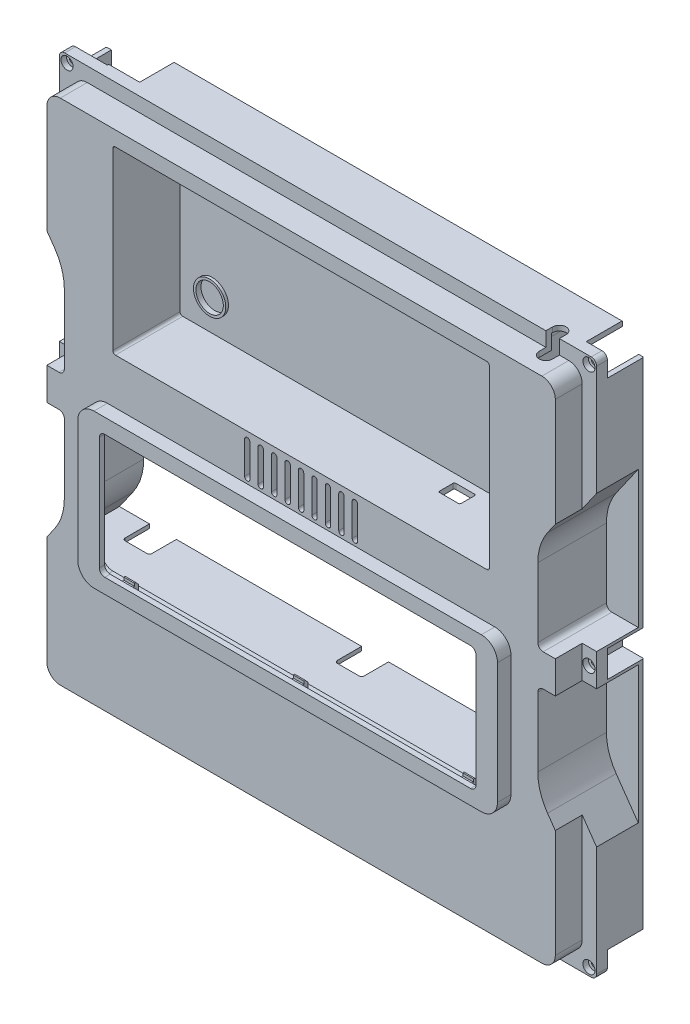
SolidWorks part; units mm, degrees
ref_plane "Front Plane" through (0, 0, 0) normal (0, 0, 1) x (1, 0, 0)
ref_plane "Top Plane" through (0, 0, 0) normal (0, 1, 0) x (1, 0, 0)
ref_plane "Right Plane" through (0, 0, 0) normal (1, 0, 0) x (0, 0, -1)
other "Configuration Table"
sketch "Sketch1" plane through (0, 0, 0) normal (0, 0, 1) x (1, 0, 0)
  line L1 (-100, 100) -> (100, 100)
  line L2 (-100, 100) -> (-100, -100)
  line L3 (-100, -100) -> (100, -100)
  line L4 (100, 100) -> (100, -100)
  line L5 (-100, 100) -> (100, -100) construction
  line L6 (-100, -100) -> (100, 100) construction
  point P0 (0, 0)
  dimension "D1" = 200
  dimension "D2" = 200
extrude "Boss-Extrude1" add sketch "Sketch1" along normal blind 17.5
sketch "Sketch2" plane through (0, 0, 17.5) normal (0, 0, 1) x (1, 0, 0)
  line L1 (-94.5, 94.5) -> (94.5, 94.5)
  line L2 (-94.5, 94.5) -> (-94.5, -94.5)
  line L3 (-94.5, -94.5) -> (94.5, -94.5)
  line L4 (94.5, 94.5) -> (94.5, -94.5)
  line L5 (-94.5, 94.5) -> (94.5, -94.5) construction
  line L6 (-94.5, -94.5) -> (94.5, 94.5) construction
  point P0 (0, 0)
  dimension "D1" = 189
  dimension "D2" = 189
extrude "Boss-Extrude2" add sketch "Sketch2" along normal blind 10
sketch "Sketch3" plane through (0, 0, 27.5) normal (0, 0, 1) x (1, 0, 0)
  line L0 (0, 0) -> (0, 94.5) construction
  line L1 (94.5, 94.5) -> (-94.5, 94.5) construction
  line L2 (-88, 33.694) -> (-88, 6)
  line L3 (-91.617, -45.1656) -> (-112.6112, -75.1484)
  line L4 (-112.6112, -75.1484) -> (-112.6112, 75.1484)
  line L5 (-112.6112, 75.1484) -> (-91.617, 45.1656)
  line L6 (-100, 100) -> (-100, -100) construction
  line L7 (112.6112, 75.1484) -> (91.617, 45.1656)
  line L8 (112.6112, -75.1484) -> (112.6112, 75.1484)
  line L9 (91.617, -45.1656) -> (112.6112, -75.1484)
  line L10 (88, 33.694) -> (88, 6)
  line L11 (-88, 6) -> (-101.9301, 6)
  line L12 (-101.9301, 6) -> (-101.9301, -6)
  line L13 (-101.9301, -6) -> (-88, -6)
  line L14 (-88, -6) -> (-88, -33.694)
  line L15 (101.9301, -6) -> (88, -6)
  line L16 (101.9301, 6) -> (101.9301, -6)
  line L17 (88, 6) -> (101.9301, 6)
  line L18 (88, -6) -> (88, -33.694)
  line L19 (-101.9301, 0) -> (-43.6967, 0) construction
  arc A2 (-88, -33.694) -> (-91.617, -45.1656) centre (-108, -33.694) cw
  arc A3 (-88, 33.694) -> (-91.617, 45.1656) centre (-108, 33.694) ccw
  arc A4 (88, 33.694) -> (91.617, 45.1656) centre (108, 33.694) cw
  arc A5 (88, -33.694) -> (91.617, -45.1656) centre (108, -33.694) ccw
  point P13 (-88, -40)
  point P16 (-88, 40)
  point P25 (88, 40)
  point P26 (88, -40)
  dimension "D5" = 20
  dimension "D1" = 80
  dimension "D2" = 35
  dimension "D3" = 35
  dimension "D4" = 12
  dimension "D6" = 12
  dimension "D7" = 40
extrude "Cut-Extrude2" cut sketch "Sketch3" against normal blind 30
sketch "Sketch4" plane through (0, 0, 27.5) normal (0, 0, 1) x (1, 0, 0)
  line L1 (-69, 89) -> (69, 89)
  line L2 (-70, 88) -> (-70, 23)
  line L3 (-69, 22) -> (69, 22)
  line L4 (70, 88) -> (70, 23)
  line L5 (-70, 89) -> (70, 22) construction
  line L6 (-70, 22) -> (70, 89) construction
  line L7 (-100, -100) -> (100, -100) construction
  arc A0 (69, 22) -> (70, 23) centre (69, 23) ccw
  arc A1 (69, 89) -> (70, 88) centre (69, 88) cw
  arc A2 (-70, 23) -> (-69, 22) centre (-69, 23) ccw
  arc A3 (-69, 89) -> (-70, 88) centre (-69, 88) ccw
  point P0 (0, 55.5)
  dimension "D4" = 1
  dimension "D1" = 67
  dimension "D2" = 140
  dimension "D3" = 122
extrude "Cut-Extrude3" cut sketch "Sketch4" against normal blind 25
sketch "Sketch5" plane through (0, 0, 27.5) normal (0, 0, 1) x (1, 0, 0)
  line L0 (-100, -100) -> (100, -100) construction
  line L1 (-72, 5) -> (72, 5)
  line L2 (-78, -1) -> (-78, -46)
  line L3 (-72, -52) -> (72, -52)
  line L4 (78, -1) -> (78, -46)
  line L5 (-78, 5) -> (78, -52) construction
  line L6 (-78, -52) -> (78, 5) construction
  arc A0 (72, -52) -> (78, -46) centre (72, -46) ccw
  arc A1 (72, 5) -> (78, -1) centre (72, -1) cw
  arc A2 (-78, -46) -> (-72, -52) centre (-72, -46) ccw
  arc A3 (-72, 5) -> (-78, -1) centre (-72, -1) ccw
  point P0 (0, -23.5)
  dimension "D4" = 6
  dimension "D1" = 156
  dimension "D2" = 57
  dimension "D3" = 48
extrude "Boss-Extrude3" add sketch "Sketch5" along normal blind 5
shell "Shell1" thickness 2
sketch "Sketch6" plane through (0, 0, 30.5) normal (0, 0, -1) x (-1, 0, 0)
  line L0 (-72, 3) -> (72, 3) construction
  line L1 (-68, -0.5) -> (68, -0.5)
  line L2 (-70, -2.5) -> (-70, -44.5)
  line L3 (-68, -46.5) -> (68, -46.5)
  line L4 (70, -2.5) -> (70, -44.5)
  line L5 (-70, -0.5) -> (70, -46.5) construction
  line L6 (-70, -46.5) -> (70, -0.5) construction
  arc A0 (-70, -44.5) -> (-68, -46.5) centre (-68, -44.5) ccw
  arc A1 (68, -46.5) -> (70, -44.5) centre (68, -44.5) ccw
  arc A2 (68, -0.5) -> (70, -2.5) centre (68, -2.5) cw
  arc A3 (-68, -0.5) -> (-70, -2.5) centre (-68, -2.5) ccw
  point P0 (0, -23.5)
  dimension "D4" = 2
  dimension "D1" = 140
  dimension "D2" = 46
  dimension "D3" = 3.5
extrude "Cut-Extrude4" cut sketch "Sketch6" against normal through all
sketch "Sketch7" plane through (0, 100, 0) normal (0, 1, 0) x (1, 0, 0)
  line L0 (-88, -10) -> (-79, -10) construction
  line L1 (-88, -8.5) -> (-79, -8.5)
  line L3 (94.5, -17.5) -> (-94.5, -17.5) construction
  line L4 (-100, -17.5) -> (-100, 0) construction
  line L8 (-89.5, -10) -> (-89.5, -13)
  line L9 (100, -17.5) -> (-100, -17.5) construction
  line L10 (-77.5, -10) -> (-77.5, -13)
  line L13 (-89.5, -13) -> (-81, -13)
  line L15 (-77.5, -13) -> (-81, -13)
  arc A0 (-88, -8.5) -> (-89.5, -10) centre (-88, -10) ccw
  arc A1 (-77.5, -10) -> (-79, -8.5) centre (-79, -10) ccw
  point P2 (-85.5, -10.5)
  dimension "D2" = 12
  dimension "D6" = 4.5
  dimension "D1" = 7.5
  dimension "D3" = 9
  dimension "D4" = 4.5
extrude "Cut-Extrude5" cut sketch "Sketch7" against normal blind 5.5
sketch "Sketch9" plane through (0, 0, 27.5) normal (0, 0, 1) x (1, 0, 0)
  line L0 (72, 5) -> (-72, 5) construction
  line L5 (0, 19) -> (0, 7) construction
  line L6 (1, 19) -> (1, 7)
  line L7 (-1, 19) -> (-1, 7)
  arc A0 (1, 19) -> (-1, 19) centre (0, 19) ccw
  arc A1 (-1, 7) -> (1, 7) centre (0, 7) ccw
  point P2 (0, 13)
  dimension "D3" = 2
  dimension "D1" = 2
  dimension "D2" = 12
extrude "Cut-Extrude6" cut sketch "Sketch9" against normal up to next
sketch "Sketch10" plane through (0, 0, 25.5) normal (0, 0, -1) x (-1, 0, 0)
  line L0 (-95.7907, -53.5) -> (-96.5907, -54.3)
  line L1 (95.9105, -53.5) -> (-95.7907, -53.5)
  line L2 (96.7105, -54.3) -> (96.7105, -55)
  line L3 (96.7105, -55) -> (-96.5907, -55)
  line L4 (-96.5907, -54.3) -> (-96.5907, -55)
  line L5 (100, -100) -> (-100, -100) construction
  line L6 (96.7105, -54.3) -> (95.9105, -53.5)
  point P0 (96.7105, -53.5)
  point P3 (-96.5907, -53.5)
  dimension "D1" = 1.5
  dimension "D2" = 45
extrude "Boss-Extrude4" add sketch "Sketch10" along normal blind 25.5
pattern_linear "LPattern1" count 5 spacing 5 along (1, 0, 0) count 5 spacing 5 along (-1, 0, 0) seed only of "Cut-Extrude6"
sketch "Sketch12" plane through (0, 100, 0) normal (0, 1, 0) x (1, 0, 0)
  line L0 (-77.5, -13) -> (-77.5, -10) construction
  line L1 (-77.5, -11.5) -> (-89.5, -11.5)
  line L2 (-77.5, -11.5) -> (-77.5, 7.4305)
  line L3 (-77.5, 7.4305) -> (-89.5, 7.4305)
  line L4 (-89.5, -11.5) -> (-89.5, 7.4305)
extrude "Cut-Extrude8" cut sketch "Sketch12" against normal blind 2
sketch "Sketch13" plane through (0, 0, 2.5) normal (0, 0, 1) x (1, 0, 0)
  line L0 (-70, 55.5) -> (70, 55.5) construction
  line L1 (-70, 88) -> (-70, 23) construction
  line L2 (70, 23) -> (70, 88) construction
  line L3 (0, 89) -> (0, 22) construction
  line L4 (69, 89) -> (-69, 89) construction
  line L5 (-69, 22) -> (69, 22) construction
  line L6 (69, 89) -> (-69, 89) construction
  line L7 (-58, 77) -> (58, 77) construction
  line L8 (-58, 77) -> (-58, 34) construction
  line L9 (-58, 34) -> (58, 34) construction
  line L10 (58, 77) -> (58, 34) construction
  line L11 (-58, 77) -> (58, 34) construction
  line L12 (-58, 34) -> (58, 77) construction
  circle A0 centre (-58, 77) radius 5.1
  circle A1 centre (58, 77) radius 5.1
  circle A2 centre (58, 34) radius 5.1
  circle A3 centre (-58, 34) radius 5.1
  circle A4 centre (-58, 77) radius 6
  circle A5 centre (-58, 34) radius 6
  circle A6 centre (58, 34) radius 6
  circle A7 centre (58, 77) radius 6
  point P12 (0, 55.5)
  dimension "D1" = 12
  dimension "D2" = 10.2
  dimension "D3" = 12
  dimension "D4" = 12
extrude "Boss-Extrude5" add sketch "Sketch13" along normal blind 1
sketch "Sketch14" plane through (0, 0, 0) normal (0, 0, -1) x (-1, 0, 0)
  line L1 (92, 108) -> (108, 108)
  line L2 (92, 108) -> (92, 92)
  line L3 (92, 92) -> (108, 92)
  line L4 (108, 108) -> (108, 92)
  line L5 (92, 108) -> (108, 92) construction
  line L6 (92, 92) -> (108, 108) construction
  line L7 (-108, 108) -> (-92, 108)
  line L8 (-108, 108) -> (-108, 92)
  line L9 (-108, 92) -> (-92, 92)
  line L10 (-92, 108) -> (-92, 92)
  line L11 (-108, 108) -> (-92, 92) construction
  line L12 (-108, 92) -> (-92, 108) construction
  line L13 (92, -92) -> (108, -92)
  line L14 (92, -92) -> (92, -108)
  line L15 (92, -108) -> (108, -108)
  line L16 (108, -92) -> (108, -108)
  line L17 (92, -92) -> (108, -108) construction
  line L18 (92, -108) -> (108, -92) construction
  line L19 (-108, -92) -> (-92, -92)
  line L20 (-108, -92) -> (-108, -108)
  line L21 (-108, -108) -> (-92, -108)
  line L22 (-92, -92) -> (-92, -108)
  line L23 (-108, -92) -> (-92, -108) construction
  line L24 (-108, -108) -> (-92, -92) construction
  line L25 (100, 100) -> (100, 57.1378) construction
  line L26 (89.5, 100) -> (100, 100) construction
  line L27 (-100, -100) -> (-100, -57.1378) construction
  line L28 (100, -100) -> (-100, -100) construction
  line L30 (-110.1437, 10.9337) -> (-92, 10.9337)
  line L31 (-110.1437, 10.9337) -> (-110.1437, -10.1129)
  line L32 (-110.1437, -10.1129) -> (-92, -10.1129)
  line L33 (-92, 10.9337) -> (-92, -10.1129)
  line L34 (92, 13.3418) -> (106.1151, 13.3418)
  line L35 (92, 13.3418) -> (92, -10.1129)
  line L36 (92, -10.1129) -> (106.1151, -10.1129)
  line L37 (106.1151, 13.3418) -> (106.1151, -10.1129)
  point P0 (100, 100)
  point P6 (-100, 100)
  point P12 (100, -100)
  point P18 (-100, -100)
  dimension "D1" = 8
  dimension "D2" = 8
  dimension "D3" = 8
  dimension "D4" = 8
extrude "Cut-Extrude9" cut sketch "Sketch14" against normal blind 13.5
sketch "Sketch15" plane through (0, 0, 15.5) normal (0, 0, -1) x (-1, 0, 0)
  line L0 (92.5, -92.5) -> (-92.5, -92.5) construction
  line L1 (-98, 98) -> (-92.5, 98)
  line L2 (-98, 98) -> (-98, 92.5)
  line L3 (-98, 92.5) -> (-92.5, 92.5)
  line L4 (-92.5, 98) -> (-92.5, 92.5)
  line L5 (98, 98) -> (92.5, 98)
  line L6 (98, 98) -> (98, 92.5)
  line L7 (98, 92.5) -> (92.5, 92.5)
  line L8 (92.5, 98) -> (92.5, 92.5)
  line L9 (98, -98) -> (92.5, -98)
  line L10 (98, -98) -> (98, -92.5)
  line L11 (98, -92.5) -> (92.5, -92.5)
  line L12 (92.5, -98) -> (92.5, -92.5)
  line L13 (-98, -98) -> (-92.5, -98)
  line L14 (-98, -98) -> (-98, -92.5)
  line L15 (-98, -92.5) -> (-92.5, -92.5)
  line L16 (-92.5, -98) -> (-92.5, -92.5)
  line L17 (92.5, -92.5) -> (-92.5, -92.5) construction
  line L19 (-100, 6) -> (-92, 6)
  line L20 (-100, 6) -> (-100, -6)
  line L21 (-100, -6) -> (-92, -6)
  line L22 (-92, 6) -> (-92, -6)
  line L23 (100, 6) -> (92, 6)
  line L24 (100, 6) -> (100, -6)
  line L25 (100, -6) -> (92, -6)
  line L26 (92, 6) -> (92, -6)
extrude "Boss-Extrude6" add sketch "Sketch15" along normal blind 2
sketch "Sketch16" plane through (0, 0, 17.5) normal (0, 0, 1) x (1, 0, 0)
  line L0 (94.5, -94.5) -> (94.5, -55) construction
  line L1 (-97, 97) -> (97, 97) construction
  line L2 (-97, 97) -> (-97, -97) construction
  line L3 (-97, -97) -> (97, -97) construction
  line L4 (97, 97) -> (97, -97) construction
  line L5 (-94.5, -94.5) -> (94.5, -94.5) construction
  line L6 (94.5, 94.5) -> (-94.5, 94.5) construction
  line L7 (-94.5, 94.5) -> (-94.5, 49.283) construction
  circle A0 centre (-97, 97) radius 1.1
  circle A1 centre (97, 97) radius 1.1
  circle A2 centre (97, -97) radius 1.1
  circle A3 centre (-97, -97) radius 1.1
  circle A4 centre (-97, 0) radius 1.1
  circle A5 centre (97, 0) radius 1.1
  dimension "D5" = 2.2
  dimension "D1" = 2.5
  dimension "D2" = 2.5
  dimension "D3" = 2.5
  dimension "D4" = 2.5
extrude "Cut-Extrude10" cut sketch "Sketch16" against normal through all
sketch "Sketch17" plane through (0, 0, 0) normal (0, 0, -1) x (-1, 0, 0)
  line L1 (86, 4) -> (92, 4)
  line L2 (86, 4) -> (86, -4)
  line L3 (86, -4) -> (92, -4)
  line L4 (92, 4) -> (92, -4)
  line L5 (-92, 4) -> (-86, 4)
  line L6 (-92, 4) -> (-92, -4)
  line L7 (-92, -4) -> (-86, -4)
  line L8 (-86, 4) -> (-86, -4)
extrude "Boss-Extrude7" add sketch "Sketch17" against normal blind 16
sketch "Sketch18" plane through (0, 0, 27.5) normal (0, 0, 1) x (1, 0, 0)
  line L0 (100, -100) -> (100, -57.1378) construction
  line L1 (-99.85, 99.85) -> (99.85, 99.85)
  line L2 (-99.85, 99.85) -> (-99.85, -99.85)
  line L3 (-99.85, -99.85) -> (99.85, -99.85)
  line L4 (99.85, 99.85) -> (99.85, -99.85)
  line L5 (-100, -100) -> (100, -100) construction
  line L6 (100, 100) -> (-100, 100) construction
  line L7 (-100, 100) -> (-100, 57.1378) construction
  line L9 (-153.5512, 137.0974) -> (153.5512, 137.0974)
  line L10 (-153.5512, 137.0974) -> (-153.5512, -137.0974)
  line L11 (-153.5512, -137.0974) -> (153.5512, -137.0974)
  line L12 (153.5512, 137.0974) -> (153.5512, -137.0974)
  line L13 (-153.5512, 137.0974) -> (153.5512, -137.0974) construction
  line L14 (-153.5512, -137.0974) -> (153.5512, 137.0974) construction
  point P12 (0, 0)
  dimension "D1" = 0.15
  dimension "D2" = 0.15
  dimension "D3" = 0.15
  dimension "D4" = 0.15
extrude "Cut-Extrude11" cut sketch "Sketch18" against normal through all both and the other way through all
sketch "Sketch20" plane through (0, 99.85, 0) normal (0, 1, 0) x (1, 0, 0)
  line L1 (-86, -13.5) -> (-98, -13.5)
  line L2 (-86, -13.5) -> (-86, 0)
  line L3 (-86, 0) -> (-98, 0)
  line L4 (-98, -13.5) -> (-98, 0)
extrude "Cut-Extrude12" cut sketch "Sketch20" against normal up to next and the other way through all
sketch "Sketch22" plane through (0, 0, 25.5) normal (0, 0, -1) x (-1, 0, 0)
  line L0 (-26, 20) -> (-26, 8)
  line L1 (69, 20) -> (-69, 20) construction
  line L2 (-24, 6) -> (24, 6)
  line L3 (26, 8) -> (26, 20)
  line L4 (69, 20) -> (20, 20) construction
  line L6 (-27, 20) -> (-27, 8)
  line L7 (-24, 5) -> (24, 5)
  line L8 (27, 8) -> (27, 20)
  line L9 (-27, 20) -> (-26, 20)
  line L10 (26, 20) -> (27, 20)
  line L11 (68, -0.5) -> (-68, -0.5) construction
  arc A0 (24, 6) -> (26, 8) centre (24, 8) ccw
  arc A1 (-26, 8) -> (-24, 6) centre (-24, 8) ccw
  arc A2 (-27, 8) -> (-24, 5) centre (-24, 8) ccw
  arc A3 (24, 5) -> (27, 8) centre (24, 8) ccw
  point P13 (26, 4)
  point P16 (-26, 4)
  dimension "D4" = 2
  dimension "D7" = 26
  dimension "D8" = 3
  dimension "D9" = 3
  dimension "D1" = 1
  dimension "D2" = 26
  dimension "D3" = 5.5
  dimension "D5" = 1
  dimension "D6" = 1
extrude "Boss-Extrude8" add sketch "Sketch22" along normal blind 12
sketch "Sketch23" plane through (0, 20, 0) normal (0, -1, 0) x (-1, 0, 0)
  line L0 (69, -25.5) -> (27, -25.5) construction
  line L1 (-42.5, -5.5) -> (-35.5, -5.5)
  line L2 (-43, -6) -> (-43, -11)
  line L3 (-42.5, -11.5) -> (-35.5, -11.5)
  line L4 (-35, -6) -> (-35, -11)
  line L5 (-43, -5.5) -> (-35, -11.5) construction
  line L6 (-43, -11.5) -> (-35, -5.5) construction
  line L7 (-26, -13.5) -> (-26, -25.5) construction
  arc A0 (-35.5, -5.5) -> (-35, -6) centre (-35.5, -6) cw
  arc A1 (-35.5, -11.5) -> (-35, -11) centre (-35.5, -11) ccw
  arc A2 (-43, -11) -> (-42.5, -11.5) centre (-42.5, -11) ccw
  arc A3 (-42.5, -5.5) -> (-43, -6) centre (-42.5, -6) ccw
  point P0 (-39, -8.5)
  dimension "D5" = 0.5
  dimension "D1" = 8
  dimension "D2" = 6
  dimension "D3" = 14
  dimension "D4" = 9
extrude "Cut-Extrude14" cut sketch "Sketch23" against normal up to next
sketch "Sketch24" plane through (0, -55, 0) normal (0, -1, 0) x (-1, 0, 0)
  line L0 (-96.0616, 0) -> (96.0616, 0) construction
  line L1 (5, 10) -> (-5, 10)
  line L2 (5, 10) -> (5, -9)
  line L3 (4, -10) -> (-4, -10)
  line L4 (-5, 10) -> (-5, -9)
  line L5 (5, 10) -> (-5, -10) construction
  line L6 (5, -10) -> (-5, 10) construction
  line L7 (0, 0) -> (0, 21.535) construction
  line L8 (-83.8576, 9.6048) -> (-73.8576, 9.6048)
  line L9 (-83.8576, 9.6048) -> (-83.8576, -9)
  line L10 (-82.8576, -10) -> (-74.8576, -10)
  line L11 (-73.8576, 9.6048) -> (-73.8576, -9)
  line L12 (73.8576, 9.6048) -> (73.8576, -9)
  line L13 (82.8576, -10) -> (74.8576, -10)
  line L14 (83.8576, 9.6048) -> (83.8576, -9)
  line L15 (83.8576, 9.6048) -> (73.8576, 9.6048)
  arc A0 (-4, -10) -> (-5, -9) centre (-4, -9) cw
  arc A1 (5, -9) -> (4, -10) centre (4, -9) cw
  arc A2 (-74.8576, -10) -> (-73.8576, -9) centre (-74.8576, -9) ccw
  arc A3 (-83.8576, -9) -> (-82.8576, -10) centre (-82.8576, -9) ccw
  arc A4 (83.8576, -9) -> (82.8576, -10) centre (82.8576, -9) cw
  arc A5 (74.8576, -10) -> (73.8576, -9) centre (74.8576, -9) cw
  point P0 (0, 0)
  point P20 (-73.8576, -10)
  point P23 (-83.8576, -10)
  point P34 (83.8576, -10)
  point P35 (73.8576, -10)
  dimension "D3" = 1
  dimension "D5" = 1
  dimension "D1" = 10
  dimension "D2" = 10
  dimension "D4" = 10
extrude "Cut-Extrude15" cut sketch "Sketch24" against normal up to next
sketch "Sketch25" plane through (0, 0, 30.5) normal (0, 0, -1) x (-1, 0, 0)
  line L0 (0, 0) -> (0, -21.9735) construction
  line L5 (-65, 2.5) -> (65, 2.5)
  line L6 (-65, 2.5) -> (-65, 1)
  line L7 (-65, 1) -> (65, 1)
  line L8 (65, 2.5) -> (65, 1)
  line L9 (-65, 2.5) -> (65, 1) construction
  line L10 (-65, 1) -> (65, 2.5) construction
  line L15 (-68, -46.5) -> (68, -46.5) construction
  line L16 (65, -49.5) -> (-65, -49.5)
  line L17 (-70, -23.5) -> (27.1802, -23.5) construction
  line L18 (-70, -2.5) -> (-70, -44.5) construction
  line L19 (68, -0.5) -> (-68, -0.5) construction
  line L20 (65, -49.5) -> (65, -48)
  line L21 (65, -48) -> (-65, -48)
  line L26 (-65, -49.5) -> (-65, -48)
  line L27 (65, -49.5) -> (-65, -48) construction
  line L28 (65, -48) -> (-65, -49.5) construction
  point P4 (0, 1.75)
  point P9 (0, -48.75)
  dimension "D1" = 1.5
  dimension "D2" = 1.5
  dimension "D3" = 130
  dimension "D4" = 1.5
  dimension "D5" = 1.5
extrude "Boss-Extrude9" add sketch "Sketch25" along normal blind 2.1
sketch "Sketch26" plane through (-65, 0, 0) normal (-1, 0, 0) x (0, 0, 1)
  line L0 (28.4, 1) -> (28.4, 0)
  line L1 (28.4, 0) -> (27.9, 0)
  line L2 (27.9, 0) -> (26.9, 1.1025)
  line L3 (26.9, 1.1025) -> (26.9, 2.5)
  line L4 (26.9, 2.5) -> (28.4, 2.5)
  line L5 (28.4, 2.5) -> (28.4, 1)
  line L6 (28.4, 1) -> (30.5, 1) construction
  line L7 (30.5, -48) -> (30.5, 1) construction
  line L8 (30.5, -23.5) -> (10.9188, -23.5) construction
  line L9 (28.4, -49.5) -> (28.4, -48)
  line L10 (26.9, -49.5) -> (28.4, -49.5)
  line L11 (26.9, -48.1025) -> (26.9, -49.5)
  line L12 (27.9, -47) -> (26.9, -48.1025)
  line L13 (28.4, -47) -> (27.9, -47)
  line L14 (28.4, -48) -> (28.4, -47)
  dimension "D1" = 1
  dimension "D2" = 0.5
  dimension "D3" = 1.5
extrude "Boss-Extrude10" add sketch "Sketch26" against normal blind 130
sketch "Sketch27" plane through (0, 0, 26.9) normal (0, 0, -1) x (-1, 0, 0)
  line L0 (-65, 2.5) -> (65, 2.5) construction
  line L1 (-61, 2.5) -> (-2, 2.5)
  line L2 (-61, 2.5) -> (-61, -49.5)
  line L3 (-61, -49.5) -> (-2, -49.5)
  line L4 (-2, 2.5) -> (-2, -49.5)
  line L5 (-65, -49.5) -> (65, -49.5) construction
  line L6 (65, 2.5) -> (65, 1.1025) construction
  line L7 (61, 2.5) -> (2, 2.5)
  line L8 (61, 2.5) -> (61, -49.5)
  line L9 (61, -49.5) -> (2, -49.5)
  line L10 (2, 2.5) -> (2, -49.5)
  line L11 (-65, 2.5) -> (-65, 1.1025) construction
  dimension "D1" = 4
  dimension "D2" = 4
  dimension "D3" = 59
  dimension "D4" = 59
extrude "Cut-Extrude16" cut sketch "Sketch27" against normal blind 3.6
sketch "Sketch31" plane through (0, 0, 0) normal (0, 0, -1) x (-1, 0, 0)
  line L0 (99.85, 56.9236) -> (99.85, 6)
  line L1 (99.85, -56.9236) -> (87.9558, -40.9839)
  line L2 (87.9558, -40.9839) -> (86.9658, -34.1155)
  line L3 (86.9658, -34.1155) -> (86.9658, 34.4794)
  line L4 (86.9658, 34.4794) -> (88.8392, 42.4561)
  line L5 (88.8392, 42.4561) -> (99.85, 56.9236)
  line L6 (99.85, 6) -> (92, 6)
  line L7 (92, 6) -> (92, -6)
  line L8 (92, -6) -> (99.85, -6)
  line L9 (99.85, -6) -> (99.85, -56.9236)
  line L10 (0, 0) -> (0, -38.0497) construction
  line L11 (-99.85, -6) -> (-99.85, -56.9236)
  line L12 (-92, -6) -> (-99.85, -6)
  line L13 (-92, 6) -> (-92, -6)
  line L14 (-99.85, 6) -> (-92, 6)
  line L15 (-88.8392, 42.4561) -> (-99.85, 56.9236)
  line L16 (-86.9658, 34.4794) -> (-88.8392, 42.4561)
  line L17 (-86.9658, -34.1155) -> (-86.9658, 34.4794)
  line L18 (-87.9558, -40.9839) -> (-86.9658, -34.1155)
  line L19 (-99.85, -56.9236) -> (-87.9558, -40.9839)
  line L20 (-99.85, 56.9236) -> (-99.85, 6)
extrude "Boss-Extrude13" add sketch "Sketch31" against normal blind 2
sketch "Sketch33" plane through (0, 0, 13.5) normal (0, 0, -1) x (-1, 0, 0)
  line L1 (-99.85, 6) -> (-92, 6)
  line L2 (-99.85, 6) -> (-99.85, 5)
  line L3 (-99.85, 5) -> (-92, 5)
  line L4 (-92, 6) -> (-92, 5)
  line L5 (-92, -6) -> (-92, 6) construction
  line L6 (-99.85, -6) -> (-92, -6)
  line L7 (-99.85, -6) -> (-99.85, -5)
  line L8 (-99.85, -5) -> (-92, -5)
  line L9 (-92, -6) -> (-92, -5)
  line L10 (0, -0.5) -> (0, -27.2849) construction
  line L11 (68, -0.5) -> (-68, -0.5) construction
  line L12 (92, -6) -> (92, -5)
  line L13 (99.85, -5) -> (92, -5)
  line L14 (99.85, -6) -> (99.85, -5)
  line L15 (99.85, -6) -> (92, -6)
  line L16 (92, 6) -> (92, 5)
  line L17 (99.85, 5) -> (92, 5)
  line L18 (99.85, 6) -> (99.85, 5)
  line L19 (99.85, 6) -> (92, 6)
  dimension "D1" = 1
  dimension "D2" = 1
extrude "Boss-Extrude19" add sketch "Sketch33" along normal blind 13.5
sketch "Sketch34" plane through (0, 0, 17.5) normal (0, 0, 1) x (1, 0, 0)
  circle A0 centre (97, 97) radius 2.25
  circle A1 centre (97, 0) radius 2.25
  circle A2 centre (97, -97) radius 2.25
  circle A3 centre (-97, -97) radius 2.25
  circle A4 centre (-97, 0) radius 2.25
  circle A5 centre (-97, 97) radius 2.25
  dimension "D1" = 4.5
extrude "Cut-Extrude18" cut sketch "Sketch34" against normal blind 2
fillet "Fillet1" radius 5 4 edges at (94.5, -94.5, 22.5) (-94.5, -94.5, 22.5) (-94.5, 94.5, 22.5) (94.5, 94.5, 22.5)
fillet "Fillet2" radius 2 4 edges at (-99.85, -99.85, 15.5) (99.85, -99.85, 15.5) (99.85, 99.85, 15.5) (-99.85, 99.85, 15.5)
fillet "Fillet3" radius 2 4 edges at (88, 6, 14.75) (88, -6, 14.75) (-88, 6, 14.75) (-88, -6, 14.75)
chamfer "Chamfer1" distance 0.2 angle 45 6 edges at (99.85, -48.5, 0) (99.85, 48.5, 0) (0, -99.85, 0) (-99.85, -48.5, 0) (-99.85, 48.5, 0) (7.25, 99.85, 0)
sketch "Sketch35" plane through (0, 0, 2.5) normal (0, 0, 1) x (1, 0, 0)
  circle A0 centre (-58, 34) radius 5.1
  circle A1 centre (-58, 77) radius 5.1
  circle A2 centre (58, 77) radius 5.1
  circle A3 centre (58, 34) radius 5.1
extrude "Cut-Extrude19" cut sketch "Sketch35" against normal blind 0.9
sketch "Sketch36" plane through (-77.5, 0, 0) normal (-1, 0, 0) x (0, 0, 1)
  line L1 (0, 98) -> (13, 98)
  line L2 (0, 98) -> (0, 99.85)
  line L3 (0, 99.85) -> (13, 99.85)
  line L4 (13, 98) -> (13, 99.85)
extrude "Cut-Extrude20" cut sketch "Sketch36" against normal blind 3
sketch "Sketch37" plane through (0, 99.85, 0) normal (0, 1, 0) x (1, 0, 0)
  line L0 (83.5, -15) -> (83.5, -20) construction
  line L1 (86, -15) -> (86, -20)
  line L2 (81, -15) -> (81, -20)
  line L3 (97.85, -17.5) -> (-97.85, -17.5) construction
  line L4 (99.85, -0.2) -> (99.85, -13.5) construction
  line L5 (89.5, -17.5) -> (-89.5, -17.5) construction
  arc A0 (86, -15) -> (81, -15) centre (83.5, -15) ccw
  arc A1 (81, -20) -> (86, -20) centre (83.5, -20) ccw
  point P2 (83.5, -17.5)
  dimension "D2" = 2.5
  dimension "D3" = 16.35
  dimension "D1" = 5
  dimension "D4" = 2.5
extrude "Cut-Extrude21" cut sketch "Sketch37" against normal blind 15
sketch "Sketch38" plane through (0, 0, 30.5) normal (0, 0, -1) x (-1, 0, 0)
  line L0 (-72, 3) -> (72, 3) construction
  line L1 (-65, 2.5) -> (-61, 2.5)
  line L2 (-65, 2.5) -> (-65, 3)
  line L3 (-65, 3) -> (-61, 3)
  line L4 (-61, 2.5) -> (-61, 3)
  line L5 (72, -50) -> (-72, -50) construction
  line L6 (-65, -49.5) -> (-61, -49.5)
  line L7 (-65, -49.5) -> (-65, -50)
  line L8 (-65, -50) -> (-61, -50)
  line L9 (-61, -49.5) -> (-61, -50)
  line L10 (-72, 3) -> (72, 3) construction
  line L11 (-2, 2.5) -> (2, 2.5)
  line L12 (-2, 2.5) -> (-2, 3)
  line L13 (-2, 3) -> (2, 3)
  line L14 (2, 2.5) -> (2, 3)
  line L15 (61, 2.5) -> (65, 2.5)
  line L16 (61, 2.5) -> (61, 3)
  line L17 (61, 3) -> (65, 3)
  line L18 (65, 2.5) -> (65, 3)
  line L20 (-2, -49.5) -> (2, -49.5)
  line L21 (-2, -49.5) -> (-2, -50)
  line L22 (-2, -50) -> (2, -50)
  line L23 (2, -49.5) -> (2, -50)
  line L24 (61, -49.5) -> (65, -49.5)
  line L25 (61, -49.5) -> (61, -50)
  line L26 (61, -50) -> (65, -50)
  line L27 (65, -49.5) -> (65, -50)
extrude "Boss-Extrude20" add sketch "Sketch38" along normal blind 3.6
sketch "Sketch39" plane through (0, -55, 0) normal (0, -1, 0) x (-1, 0, 0)
  line L1 (94.5, -25.5) -> (96.7105, -25.5)
  line L2 (94.5, -25.5) -> (94.5, -17.5)
  line L3 (94.5, -17.5) -> (96.7105, -17.5)
  line L4 (96.7105, -25.5) -> (96.7105, -17.5)
  line L5 (-94.5, -25.5) -> (-96.5907, -25.5)
  line L6 (-94.5, -25.5) -> (-94.5, -17.5)
  line L7 (-94.5, -17.5) -> (-96.5907, -17.5)
  line L8 (-96.5907, -25.5) -> (-96.5907, -17.5)
extrude "Cut-Extrude22" cut sketch "Sketch39" against normal blind 2
